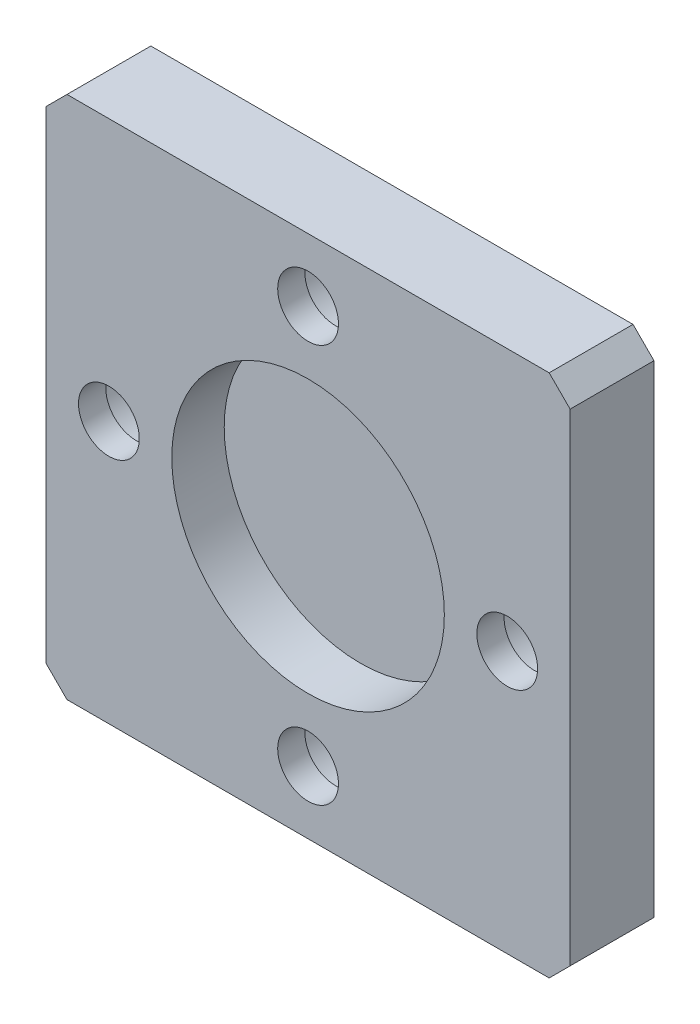
SolidWorks part; units mm, degrees
material "6061Al"
ref_plane "前视基准面" through (0, 0, 0) normal (0, 0, 1) x (1, 0, 0)
ref_plane "上视基准面" through (0, 0, 0) normal (0, 1, 0) x (1, 0, 0)
ref_plane "右视基准面" through (0, 0, 0) normal (1, 0, 0) x (0, 0, -1)
sketch "草图1" plane through (0, 0, 0) normal (0, 0, 1) x (1, 0, 0)
  line L1 (-25, -25) -> (25, -25)
  line L2 (-25, -25) -> (-25, 25)
  line L3 (-25, 25) -> (25, 25)
  line L4 (25, -25) -> (25, 25)
  line L5 (-25, -25) -> (25, 25) construction
  line L6 (-25, 25) -> (25, -25) construction
  point P0 (0, 0)
  dimension "D1" = 50
  dimension "D2" = 50
extrude "凸台-拉伸1" add sketch "草图1" along normal mid plane 8
sketch "草图2" plane through (0, 0, 4) normal (0, 0, 1) x (1, 0, 0)
  circle A0 centre (0, 0) radius 13
  dimension "D1" = 26
extrude "切除-拉伸1" cut sketch "草图2" against normal blind 5
hole_wizard "M5 六角凹头螺钉的柱形沉头孔1" positions "草图6" profile "草图5" counterbore size "M5" standard "ISO" end condition through all
sketch "草图6" plane through (0, 0, -4) normal (0, 0, 1) x (1, 0, 0)
  line L1 (-19, -19) -> (19, -19)
  line L2 (-19, -19) -> (-19, 19)
  line L3 (-19, 19) -> (19, 19)
  line L4 (19, -19) -> (19, 19)
  line L5 (-19, -19) -> (19, 19) construction
  line L6 (-19, 19) -> (19, -19) construction
  line L7 (-25, 25) -> (-25, -25) construction
  point P45 (0, 19)
  point P47 (19, 0)
  point P49 (0, -19)
  point P51 (-19, 0)
  point P53 (0, 0)
  dimension "D1" = 6
sketch "草图5" plane through (-19, 0, -4) normal (1, 0, 0) x (0, 1, 0)
  line L0 (0, 0) -> (0, 8)
  line L1 (0, 8) -> (2.9, 8)
  line L3 (2.9, 8) -> (2.9, 5.4)
  line L4 (2.9, 5.4) -> (5, 5.4)
  line L5 (5, 5.4) -> (5, 0)
  line L7 (5, 0) -> (0, 0)
  line L11 (0, -6.35) -> (0, 107.95) construction
  dimension "通孔孔直径" = 5.8
  dimension "通孔孔深度" = 8
  dimension "柱形沉头孔直径" = 10
  dimension "柱形沉头孔深度" = 5.4
chamfer "倒角1" distance 2 angle 45 4 edges at (-25, -25, 0) (25, -25, 0) (25, 25, 0) (-25, 25, 0)
sketch "草图7" plane through (0, 0, 4) normal (0, 0, 1) x (1, 0, 0)
  circle A0 centre (0, 0) radius 13 construction
  circle A1 centre (0, 0) radius 13
  circle A2 centre (0, 0) radius 14
  dimension "D1" = 28
extrude "凸台-拉伸2" [suppressed] add sketch "草图7" against normal blind 3.2
